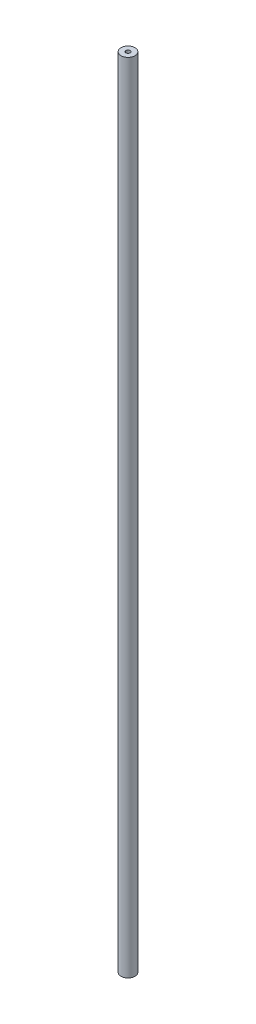
SolidWorks part; units mm, degrees
ref_plane "前视基准面" through (0, 0, 0) normal (0, 0, 1) x (1, 0, 0)
ref_plane "上视基准面" through (0, 0, 0) normal (0, 1, 0) x (1, 0, 0)
ref_plane "右视基准面" through (0, 0, 0) normal (1, 0, 0) x (0, 0, -1)
sketch "草图1" plane through (0, 0, 0) normal (0, 1, 0) x (1, 0, 0)
  circle A0 centre (0, 0) radius 20
  dimension "D1" = 40
extrude "凸台-拉伸1" add sketch "草图1" along normal blind 2286
hole_wizard "M14 螺纹孔1" positions "草图2" profile "草图3" tap size "M14" standard "GB"
sketch "草图2" plane through (0, 2286, 0) normal (0, 1, 0) x (1, 0, 0)
  point P0 (0, 0)
sketch "草图3" plane through (0, 2286, 0) normal (1, 0, 0) x (0, 0, 1)
  line L0 (0, 0) -> (0, 37.6052)
  line L1 (0, 37.6052) -> (6, 34)
  line L2 (6, 34) -> (6, 0)
  line L5 (6, 0) -> (0, 0)
  line L10 (0, 37.6052) -> (-6, 34) construction
  line L11 (0, -6.35) -> (0, 107.95) construction
  dimension "螺纹孔钻头直径" = 12
  dimension "螺纹孔钻头深度" = 34
  dimension "导头角度" = 118
cosmetic thread "孔螺蚊线1" parameters "D1"=28, "D2"=14
hole_wizard "M14 螺纹孔2" positions "草图4" profile "草图5" tap size "M14" standard "GB"
sketch "草图4" plane through (0, 0, 0) normal (0, -1, 0) x (-1, 0, 0)
  point P0 (0, 0)
sketch "草图5" plane through (0, 0, 0) normal (1, 0, 0) x (0, 0, -1)
  line L0 (0, 0) -> (0, 37.6052)
  line L1 (0, 37.6052) -> (6, 34)
  line L2 (6, 34) -> (6, 0)
  line L5 (6, 0) -> (0, 0)
  line L10 (0, 37.6052) -> (-6, 34) construction
  line L11 (0, -6.35) -> (0, 107.95) construction
  dimension "螺纹孔钻头直径" = 12
  dimension "螺纹孔钻头深度" = 34
  dimension "导头角度" = 118
cosmetic thread "孔螺蚊线2" parameters "D1"=28, "D2"=14
